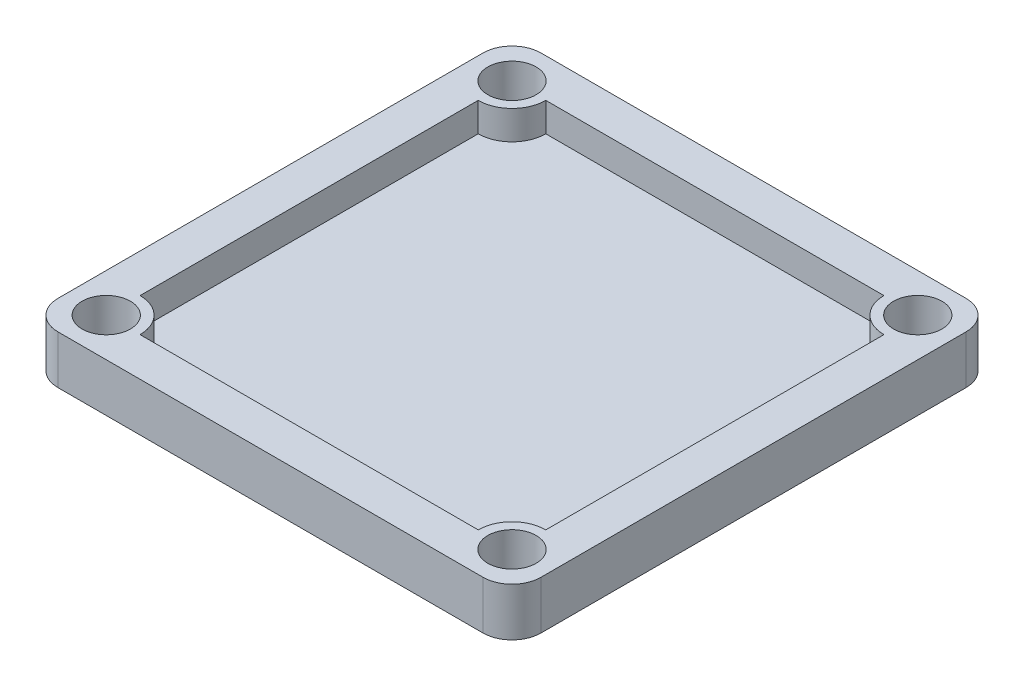
from build123d import *

# Parameters (mm, degrees)
BOSS_EXTRUDE1_DEPTH = 50
CUT_EXTRUDE1_DEPTH  = 30
CUT_EXTRUDE2_REACH  = 359.071
SKETCH3_R           = 25


with BuildPart() as part:
    # Sketch1 → Boss-Extrude1 (new body)
    with BuildSketch(Plane(origin=(0, 0, 0), x_dir=(1, 0, 0), z_dir=(0, 1, 0))):
        with BuildLine():
            Line((-220, -250), (220, -250))
            ThreePointArc((220, -250), (241.213203436, -241.213203436), (250, -220))
            Line((250, -220), (250, 220))
            ThreePointArc((250, 220), (241.213203436, 241.213203436), (220, 250))
            Line((220, 250), (-220, 250))
            ThreePointArc((-220, 250), (-241.213203436, 241.213203436), (-250, 220))
            Line((-250, 220), (-250, -220))
            ThreePointArc((-250, -220), (-241.213203436, -241.213203436), (-220, -250))
        make_face()
    extrude(amount=BOSS_EXTRUDE1_DEPTH)

    # Sketch2 → Cut-Extrude1 (cut)
    with BuildSketch(Plane(origin=(0, 50, 0), x_dir=(1, 0, 0), z_dir=(0, 1, 0))):
        with BuildLine():
            Line((-175, -210), (175, -210))
            ThreePointArc((175, -210), (185.251262658, -185.251262658), (210, -175))
            Line((210, -175), (210, 175))
            ThreePointArc((210, 175), (185.251262658, 185.251262658), (175, 210))
            Line((175, 210), (-175, 210))
            ThreePointArc((-175, 210), (-185.251262658, 185.251262658), (-210, 175))
            Line((-210, 175), (-210, -175))
            ThreePointArc((-210, -175), (-185.251262658, -185.251262658), (-175, -210))
        make_face()
    extrude(amount=-CUT_EXTRUDE1_DEPTH, mode=Mode.SUBTRACT)

    # Sketch3 → Cut-Extrude2 (cut, up to next)
    with BuildSketch(Plane(origin=(0, 50, 0), x_dir=(1, 0, 0), z_dir=(0, 1, 0)), mode=Mode.PRIVATE) as cut_extrude2_sk1:
        with Locations(Location((-210, 210, 0), (0, 0, 270))):
            Circle(SKETCH3_R)
    cut_extrude2_tool1 = extrude(cut_extrude2_sk1.sketch, amount=-CUT_EXTRUDE2_REACH, mode=Mode.PRIVATE) & part.part
    # Sketch3 → Cut-Extrude2 (cut, up to next)
    with BuildSketch(Plane(origin=(0, 50, 0), x_dir=(1, 0, 0), z_dir=(0, 1, 0)), mode=Mode.PRIVATE) as cut_extrude2_sk2:
        with Locations(Location((210, 210, 0), (0, 0, 90))):
            Circle(SKETCH3_R)
    cut_extrude2_tool2 = extrude(cut_extrude2_sk2.sketch, amount=-CUT_EXTRUDE2_REACH, mode=Mode.PRIVATE) & part.part
    # Sketch3 → Cut-Extrude2 (cut, up to next)
    with BuildSketch(Plane(origin=(0, 50, 0), x_dir=(1, 0, 0), z_dir=(0, 1, 0)), mode=Mode.PRIVATE) as cut_extrude2_sk3:
        with Locations(Location((210, -210, 0), (0, 0, 270))):
            Circle(SKETCH3_R)
    cut_extrude2_tool3 = extrude(cut_extrude2_sk3.sketch, amount=-CUT_EXTRUDE2_REACH, mode=Mode.PRIVATE) & part.part
    # Sketch3 → Cut-Extrude2 (cut, up to next)
    with BuildSketch(Plane(origin=(0, 50, 0), x_dir=(1, 0, 0), z_dir=(0, 1, 0)), mode=Mode.PRIVATE) as cut_extrude2_sk4:
        with Locations(Location((-210, -210, 0), (0, 0, 90))):
            Circle(SKETCH3_R)
    cut_extrude2_tool4 = extrude(cut_extrude2_sk4.sketch, amount=-CUT_EXTRUDE2_REACH, mode=Mode.PRIVATE) & part.part
    add(cut_extrude2_tool1.solids().sort_by_distance((-210, 50, -210))[0], mode=Mode.SUBTRACT)
    add(cut_extrude2_tool2.solids().sort_by_distance((210, 50, -210))[0], mode=Mode.SUBTRACT)
    add(cut_extrude2_tool3.solids().sort_by_distance((210, 50, 210))[0], mode=Mode.SUBTRACT)
    add(cut_extrude2_tool4.solids().sort_by_distance((-210, 50, 210))[0], mode=Mode.SUBTRACT)


solid = part.part
